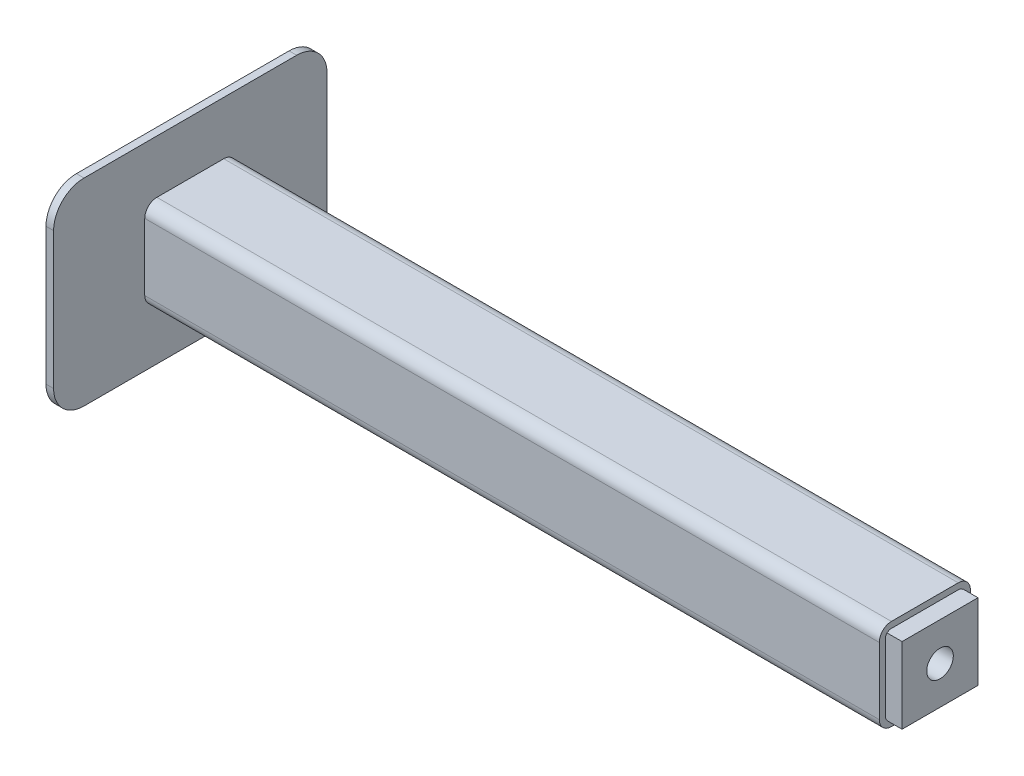
SolidWorks part; units mm, degrees
ref_plane "前视基准面" through (0, 0, 0) normal (0, 0, 1) x (1, 0, 0)
ref_plane "上视基准面" through (0, 0, 0) normal (0, 1, 0) x (1, 0, 0)
ref_plane "右视基准面" through (0, 0, 0) normal (1, 0, 0) x (0, 0, -1)
sketch "草图1" plane through (0, 0, 0) normal (0, 0, 1) x (1, 0, 0)
  line L0 (0, 0) -> (483.5, 0)
  dimension "D1" = 483.5
other "冷弯空心方管gb∕t6728-2002 60 X 60 X 4(1)"
ref_plane "基准面1" through (0, 0, 0) normal (1, 0, 0) x (0, 1, 0)
sketch "Sketch1" plane through (0, 0, 0) normal (1, 0, 0) x (0, 1, 0)
  line L0 (-22, -26) -> (22, -26)
  line L1 (-26, -22) -> (-26, 22)
  line L2 (22, 26) -> (-22, 26)
  line L3 (26, 22) -> (26, -22)
  line L4 (-22, -30) -> (22, -30)
  line L5 (-30, -22) -> (-30, 22)
  line L6 (22, 30) -> (-22, 30)
  line L7 (30, 22) -> (30, -22)
  arc A0 (30, 22) -> (22, 30) centre (22, 22) ccw
  arc A1 (22, -30) -> (30, -22) centre (22, -22) ccw
  arc A2 (-30, -22) -> (-22, -30) centre (-22, -22) ccw
  arc A3 (-22, 30) -> (-30, 22) centre (-22, 22) ccw
  arc A4 (-22, 26) -> (-26, 22) centre (-22, 22) ccw
  arc A5 (26, 22) -> (22, 26) centre (22, 22) ccw
  arc A6 (22, -26) -> (26, -22) centre (22, -22) ccw
  arc A7 (-26, -22) -> (-22, -26) centre (-22, -22) ccw
  point P0 (-30, 0)
  point P1 (30, 0)
  point P2 (0, 30)
  point P3 (0, -30)
  point P4 (0, 0)
  point P5 (-30, -30)
  point P6 (30, -30)
  point P7 (30, 30)
  point P8 (-30, 30)
  point P33 (0, 0)
  dimension "D1" = 8
  dimension "Thickness" = 4
  dimension "V_leg" = 60
sketch "草图3" plane through (0, 0, 0) normal (-1, 0, 0) x (0, 0, 1)
  line L0 (0, 65) -> (0, -65) construction
  line L1 (-70, 65) -> (70, 65)
  line L2 (-90, 45) -> (-90, -45)
  line L3 (-70, -65) -> (70, -65)
  line L4 (90, 45) -> (90, -45)
  line L5 (-90, 65) -> (90, -65) construction
  line L6 (-90, -65) -> (90, 65) construction
  arc A0 (70, 65) -> (90, 45) centre (70, 45) cw
  arc A1 (70, -65) -> (90, -45) centre (70, -45) ccw
  arc A2 (-90, -45) -> (-70, -65) centre (-70, -45) ccw
  arc A3 (-70, 65) -> (-90, 45) centre (-70, 45) ccw
  point P0 (0, 0)
  dimension "D3" = 20
  dimension "D1" = 130
  dimension "D2" = 180
extrude "凸台-拉伸1" add sketch "草图3" along normal blind 5 separate body
sketch "草图6" plane through (483.5, 0, 0) normal (1, 0, 0) x (0, 0, -1)
  line L1 (-25, 25) -> (25, 25)
  line L2 (-25, 25) -> (-25, -25)
  line L3 (-25, -25) -> (25, -25)
  line L4 (25, 25) -> (25, -25)
  line L5 (-25, 25) -> (25, -25) construction
  line L6 (-25, -25) -> (25, 25) construction
  point P0 (0, 0)
  dimension "D1" = 50
  dimension "D2" = 50
extrude "凸台-拉伸2" add sketch "草图6" along normal blind 10 and the other way blind 15 separate body
hole_wizard "M20 螺纹孔1" positions "草图7" profile "草图8" tap size "M20" standard "GB"
sketch "草图7" plane through (493.5, 0, 0) normal (1, 0, 0) x (0, 0, -1)
  point P0 (0, 0)
sketch "草图8" plane through (493.5, 0, 0) normal (0, 1, 0) x (0, 0, -1)
  line L0 (0, 0) -> (0, 57.7575)
  line L1 (0, 57.7575) -> (8.75, 52.5)
  line L2 (8.75, 52.5) -> (8.75, 0)
  line L5 (8.75, 0) -> (0, 0)
  line L10 (0, 57.7575) -> (-8.75, 52.5) construction
  line L11 (0, -6.35) -> (0, 107.95) construction
  dimension "螺纹孔钻头直径" = 17.5
  dimension "螺纹孔钻头深度" = 52.5
  dimension "导头角度" = 118
cosmetic thread "孔螺蚊线1" parameters "D1"=40, "D2"=20
